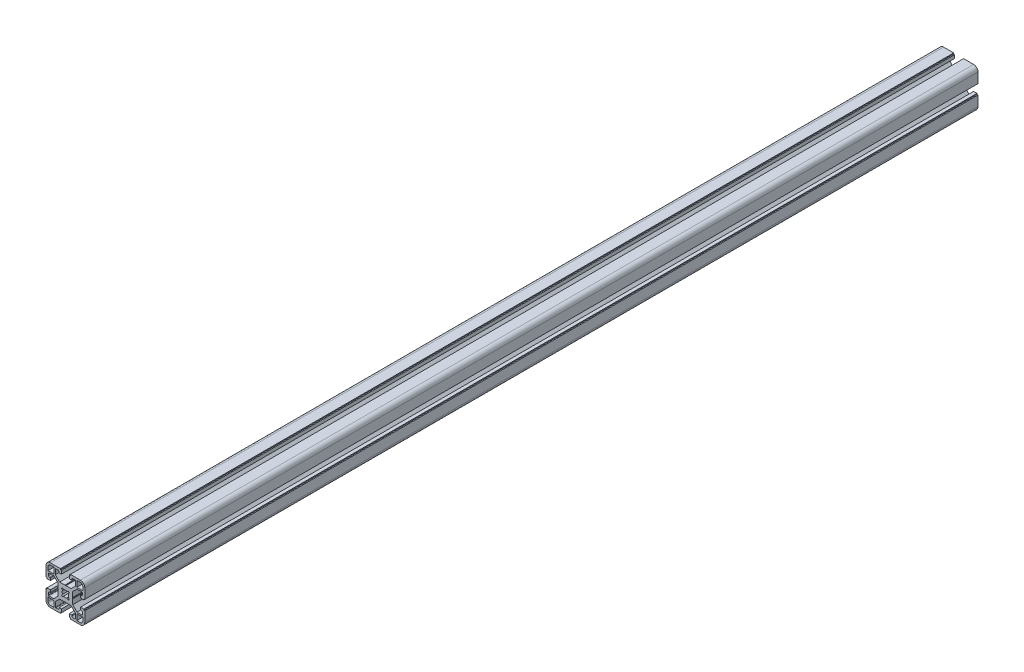
from build123d import *

# Parameters (mm, degrees)
EXTRUDE_1_DEPTH = 922


with BuildPart() as part:
    # 草图1 → 凸台-拉伸1 (new body)
    with BuildSketch(Plane.XY):
        with BuildLine():
            Line((-18.9995, -4.100341675), (-18.9995, -5.100341675))
            Line((-18.9995, -5.100341675), (-19.9995, -5.100341675))
            Line((-19.9995, -5.100341675), (-19.9995, -15.500341675))
            ThreePointArc((-19.9995, -15.500341675), (-18.681480515, -18.682322191), (-15.4995, -20.000341675))
            Line((-15.4995, -20.000341675), (-5.0995, -20.000341675))
            Line((-5.0995, -20.000341675), (-5.0995, -19.000341675))
            Line((-5.0995, -19.000341675), (-4.0995, -19.000341675))
            Line((-4.0995, -19.000341675), (-4.0995, -15.500341675))
            Line((-4.0995, -15.500341675), (-6.5995, -15.500341675))
            Line((-6.5995, -15.500341675), (-6.5995, -16.500341675))
            ThreePointArc((-6.5995, -16.500341675), (-6.892393219, -17.207448457), (-7.5995, -17.500341675))
            Line((-7.5995, -17.500341675), (-9.7995, -17.500341675))
            ThreePointArc((-9.7995, -17.500341675), (-10.153053391, -17.353895066), (-10.2995, -17.000341675))
            Line((-10.2995, -17.000341675), (-10.2995, -11.997341675))
            Line((-10.2995, -11.997341675), (-5.9025, -7.600341675))
            Line((-5.9025, -7.600341675), (-0.5195, -7.600341675))
            Line((-0.5195, -7.600341675), (0.0005, -7.300341675))
            Line((0.0005, -7.300341675), (0.5195, -7.600341675))
            Line((0.5195, -7.600341675), (5.9035, -7.600341675))
            Line((5.9035, -7.600341675), (10.3005, -11.997341675))
            Line((10.3005, -11.997341675), (10.3005, -17.000341675))
            ThreePointArc((10.3005, -17.000341675), (10.154053391, -17.353895066), (9.8005, -17.500341675))
            Line((9.8005, -17.500341675), (7.6005, -17.500341675))
            ThreePointArc((7.6005, -17.500341675), (6.893393219, -17.207448457), (6.6005, -16.500341675))
            Line((6.6005, -16.500341675), (6.6005, -15.500341675))
            Line((6.6005, -15.500341675), (4.1005, -15.500341675))
            Line((4.1005, -15.500341675), (4.1005, -19.000341675))
            Line((4.1005, -19.000341675), (5.1005, -19.000341675))
            Line((5.1005, -19.000341675), (5.1005, -20.000341675))
            Line((5.1005, -20.000341675), (15.5005, -20.000341675))
            ThreePointArc((15.5005, -20.000341675), (18.682480515, -18.682322191), (20.0005, -15.500341675))
            Line((20.0005, -15.500341675), (20.0005, -5.100341675))
            Line((20.0005, -5.100341675), (19.0005, -5.100341675))
            Line((19.0005, -5.100341675), (19.0005, -4.100341675))
            Line((19.0005, -4.100341675), (15.5005, -4.100341675))
            Line((15.5005, -4.100341675), (15.5005, -6.600341675))
            Line((15.5005, -6.600341675), (16.5005, -6.600341675))
            ThreePointArc((16.5005, -6.600341675), (17.207606781, -6.893234894), (17.5005, -7.600341675))
            Line((17.5005, -7.600341675), (17.5005, -9.800341675))
            ThreePointArc((17.5005, -9.800341675), (17.354053391, -10.153895066), (17.0005, -10.300341675))
            Line((17.0005, -10.300341675), (11.9975, -10.300341675))
            Line((11.9975, -10.300341675), (7.6005, -5.903341675))
            Line((7.6005, -5.903341675), (7.6005, -0.520341675))
            Line((7.6005, -0.520341675), (7.3005, -0.000341675))
            Line((7.3005, -0.000341675), (7.6005, 0.519658325))
            Line((7.6005, 0.519658325), (7.6005, 5.902658325))
            Line((7.6005, 5.902658325), (11.9975, 10.299658325))
            Line((11.9975, 10.299658325), (17.0005, 10.299658325))
            ThreePointArc((17.0005, 10.299658325), (17.354053391, 10.153211715), (17.5005, 9.799658325))
            Line((17.5005, 9.799658325), (17.5005, 7.599658325))
            ThreePointArc((17.5005, 7.599658325), (17.207606781, 6.892551543), (16.5005, 6.599658325))
            Line((16.5005, 6.599658325), (15.5005, 6.599658325))
            Line((15.5005, 6.599658325), (15.5005, 4.099658325))
            Line((15.5005, 4.099658325), (19.0005, 4.099658325))
            Line((19.0005, 4.099658325), (19.0005, 5.099658325))
            Line((19.0005, 5.099658325), (20.0005, 5.099658325))
            Line((20.0005, 5.099658325), (20.0005, 15.499658325))
            ThreePointArc((20.0005, 15.499658325), (18.682480515, 18.68163884), (15.5005, 19.999658325))
            Line((15.5005, 19.999658325), (5.1005, 19.999658325))
            Line((5.1005, 19.999658325), (5.1005, 18.999658325))
            Line((5.1005, 18.999658325), (4.1005, 18.999658325))
            Line((4.1005, 18.999658325), (4.1005, 15.499658325))
            Line((4.1005, 15.499658325), (6.6005, 15.499658325))
            ThreePointArc((6.6005, 15.499658325), (6.393348977, 15.999658325), (6.6005, 16.499658325))
            ThreePointArc((6.6005, 16.499658325), (6.893393219, 17.206765106), (7.6005, 17.499658325))
            Line((7.6005, 17.499658325), (9.8005, 17.499658325))
            ThreePointArc((9.8005, 17.499658325), (10.154053391, 17.353211715), (10.3005, 16.999658325))
            Line((10.3005, 16.999658325), (10.3005, 11.996658325))
            Line((10.3005, 11.996658325), (5.9035, 7.599658325))
            Line((5.9035, 7.599658325), (0.5195, 7.599658325))
            Line((0.5195, 7.599658325), (0.0005, 7.299658325))
            Line((0.0005, 7.299658325), (-0.5195, 7.599658325))
            Line((-0.5195, 7.599658325), (-5.9025, 7.599658325))
            Line((-5.9025, 7.599658325), (-10.2995, 11.996658325))
            Line((-10.2995, 11.996658325), (-10.2995, 16.999658325))
            ThreePointArc((-10.2995, 16.999658325), (-10.153053391, 17.353211715), (-9.7995, 17.499658325))
            Line((-9.7995, 17.499658325), (-7.5995, 17.499658325))
            ThreePointArc((-7.5995, 17.499658325), (-6.892393219, 17.206765106), (-6.5995, 16.499658325))
            Line((-6.5995, 16.499658325), (-6.5995, 15.499658325))
            Line((-6.5995, 15.499658325), (-4.0995, 15.499658325))
            Line((-4.0995, 15.499658325), (-4.0995, 18.999658325))
            Line((-4.0995, 18.999658325), (-5.0995, 18.999658325))
            Line((-5.0995, 18.999658325), (-5.0995, 19.999658325))
            Line((-5.0995, 19.999658325), (-15.4995, 19.999658325))
            ThreePointArc((-15.4995, 19.999658325), (-18.681480515, 18.68163884), (-19.9995, 15.499658325))
            Line((-19.9995, 15.499658325), (-19.9995, 5.099658325))
            Line((-19.9995, 5.099658325), (-18.9995, 5.099658325))
            Line((-18.9995, 5.099658325), (-18.9995, 4.099658325))
            Line((-18.9995, 4.099658325), (-15.4995, 4.099658325))
            Line((-15.4995, 4.099658325), (-15.4995, 6.599658325))
            Line((-15.4995, 6.599658325), (-16.4995, 6.599658325))
            ThreePointArc((-16.4995, 6.599658325), (-17.206606781, 6.892551543), (-17.4995, 7.599658325))
            Line((-17.4995, 7.599658325), (-17.4995, 9.799658325))
            ThreePointArc((-17.4995, 9.799658325), (-17.353053391, 10.153211715), (-16.9995, 10.299658325))
            Line((-16.9995, 10.299658325), (-11.9965, 10.299658325))
            Line((-11.9965, 10.299658325), (-7.5995, 5.902658325))
            Line((-7.5995, 5.902658325), (-7.5995, 0.519658325))
            Line((-7.5995, 0.519658325), (-7.2995, -0.000341675))
            Line((-7.2995, -0.000341675), (-7.5995, -0.520341675))
            Line((-7.5995, -0.520341675), (-7.5995, -5.903341675))
            Line((-7.5995, -5.903341675), (-11.9965, -10.300341675))
            Line((-11.9965, -10.300341675), (-16.9995, -10.300341675))
            ThreePointArc((-16.9995, -10.300341675), (-17.353053391, -10.153895066), (-17.4995, -9.800341675))
            Line((-17.4995, -9.800341675), (-17.4995, -7.600341675))
            ThreePointArc((-17.4995, -7.600341675), (-17.206606781, -6.893234894), (-16.4995, -6.600341675))
            Line((-16.4995, -6.600341675), (-15.4995, -6.600341675))
            Line((-15.4995, -6.600341675), (-15.4995, -4.100341675))
            Line((-15.4995, -4.100341675), (-18.9995, -4.100341675))
        make_face()
        with BuildLine():
            Line((15.5005, -18.000341675), (11.8005, -18.000341675))
            Line((11.8005, -18.000341675), (11.8005, -11.800341675))
            Line((11.8005, -11.800341675), (18.0005, -11.800341675))
            Line((18.0005, -11.800341675), (18.0005, -15.500341675))
            ThreePointArc((18.0005, -15.500341675), (17.268266953, -17.268108628), (15.5005, -18.000341675))
        make_face(mode=Mode.SUBTRACT)
        with BuildLine():
            Line((18.0005, 11.799658325), (11.8005, 11.799658325))
            Line((11.8005, 11.799658325), (11.8005, 17.999658325))
            Line((11.8005, 17.999658325), (15.5005, 17.999658325))
            ThreePointArc((15.5005, 17.999658325), (17.268266953, 17.267425278), (18.0005, 15.499658325))
            Line((18.0005, 15.499658325), (18.0005, 11.799658325))
        make_face(mode=Mode.SUBTRACT)
        with BuildLine():
            Line((-1.8145, -2.875341675), (-3.004391671, -4.066450004))
            Line((-3.004391671, -4.066450004), (-4.065608329, -3.005233346))
            Line((-4.065608329, -3.005233346), (-2.8745, -1.815341675))
            ThreePointArc((-2.8745, -1.815341675), (-3.399473913, -0.000341675), (-2.8745, 1.814658325))
            Line((-2.8745, 1.814658325), (-4.064391671, 3.005766654))
            Line((-4.064391671, 3.005766654), (-3.004391671, 4.065766654))
            Line((-3.004391671, 4.065766654), (-1.8145, 2.874658325))
            ThreePointArc((-1.8145, 2.874658325), (0, 3.399316649), (1.8145, 2.874658325))
            Line((1.8145, 2.874658325), (3.0055, 4.065658325))
            Line((3.0055, 4.065658325), (4.066608329, 3.004549996))
            Line((4.066608329, 3.004549996), (2.8755, 1.814658325))
            ThreePointArc((2.8755, 1.814658325), (3.400473913, -0.000341675), (2.8755, -1.815341675))
            Line((2.8755, -1.815341675), (4.066608329, -3.005233346))
            Line((4.066608329, -3.005233346), (3.0055, -4.066341675))
            Line((3.0055, -4.066341675), (1.8145, -2.875341675))
            ThreePointArc((1.8145, -2.875341675), (0, -3.4), (-1.8145, -2.875341675))
        make_face(mode=Mode.SUBTRACT)
        with BuildLine():
            Line((-17.9995, -15.500341675), (-17.9995, -11.800341675))
            Line((-17.9995, -11.800341675), (-11.7995, -11.800341675))
            Line((-11.7995, -11.800341675), (-11.7995, -18.000341675))
            Line((-11.7995, -18.000341675), (-15.4995, -18.000341675))
            ThreePointArc((-15.4995, -18.000341675), (-17.267266953, -17.268108628), (-17.9995, -15.500341675))
        make_face(mode=Mode.SUBTRACT)
        with BuildLine():
            Line((-11.7995, 17.999658325), (-11.7995, 11.799658325))
            Line((-11.7995, 11.799658325), (-17.9995, 11.799658325))
            Line((-17.9995, 11.799658325), (-17.9995, 15.499658325))
            ThreePointArc((-17.9995, 15.499658325), (-17.267266953, 17.267425278), (-15.4995, 17.999658325))
            Line((-15.4995, 17.999658325), (-11.7995, 17.999658325))
        make_face(mode=Mode.SUBTRACT)
    extrude(amount=-EXTRUDE_1_DEPTH)


solid = part.part
